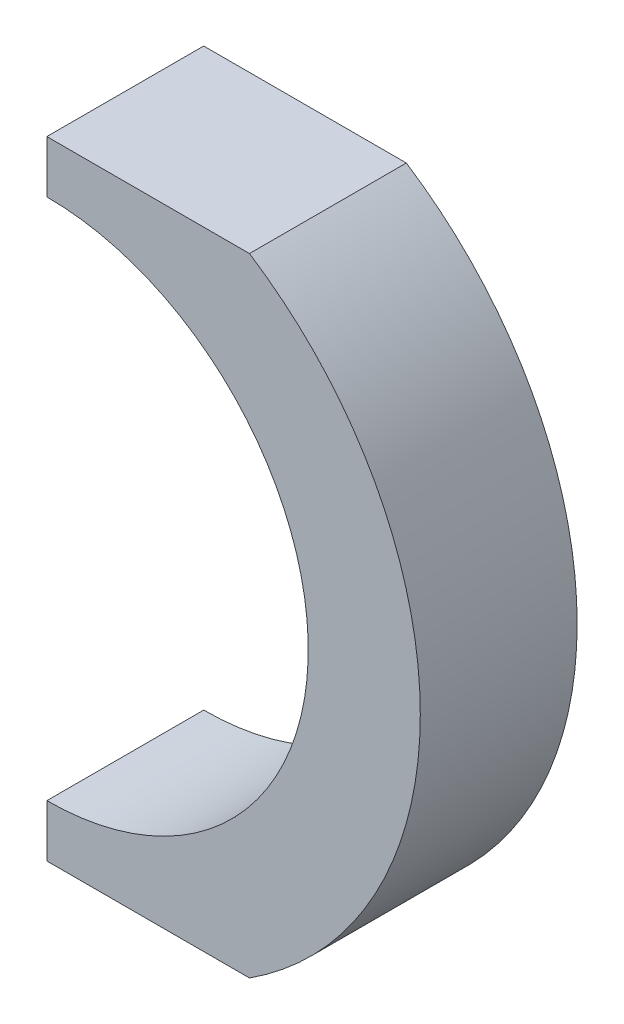
SolidWorks part; units mm, degrees
material "Q345"
ref_plane "前视基准面" through (0, 0, 0) normal (0, 0, 1) x (1, 0, 0)
ref_plane "上视基准面" through (0, 0, 0) normal (0, 1, 0) x (1, 0, 0)
ref_plane "右视基准面" through (0, 0, 0) normal (1, 0, 0) x (0, 0, -1)
sketch "草图1" plane through (0, 0, 0) normal (0, 0, 1) x (1, 0, 0)
  circle A0 centre (0, 0) radius 100
  dimension "D1" = 200
extrude "凸台-拉伸1" add sketch "草图1" along normal blind 42
sketch "草图2" plane through (0, 0, 42) normal (0, 0, 1) x (1, 0, 0)
  line L0 (0, 0) -> (-100, 0) construction
  line L1 (-54.2586, 84) -> (54.2586, 84)
  line L2 (-54.2586, -84) -> (54.2586, -84)
  circle A0 centre (0, 0) radius 100 construction
  arc A1 (-54.2586, -84) -> (54.2586, -84) centre (0, 0) ccw
  arc A2 (54.2586, 84) -> (-54.2586, 84) centre (0, 0) ccw
  dimension "D1" = 168
extrude "切除-拉伸1" cut sketch "草图2" against normal through all
sketch "草图3" plane through (0, 0, 42) normal (0, 0, 1) x (1, 0, 0)
  line L0 (100, 0) -> (70, 0) construction
  line L1 (0, 70) -> (0, 84)
  line L2 (-54.2586, 84) -> (54.2586, 84) construction
  line L3 (0, -70) -> (0, -84)
  line L4 (54.2586, -84) -> (-54.2586, -84) construction
  line L5 (0, -84) -> (-54.2586, -84)
  line L6 (-54.2586, 84) -> (0, 84)
  arc A0 (54.2586, -84) -> (54.2586, 84) centre (0, 0) ccw construction
  arc A1 (0, -70) -> (0, 70) centre (0, 0) ccw
  arc A2 (-54.2586, 84) -> (-54.2586, -84) centre (0, 0) ccw construction
  arc A3 (-54.2586, 84) -> (-54.2586, -84) centre (0, 0) ccw
  dimension "D1" = 30
extrude "切除-拉伸2" cut sketch "草图3" against normal through all
